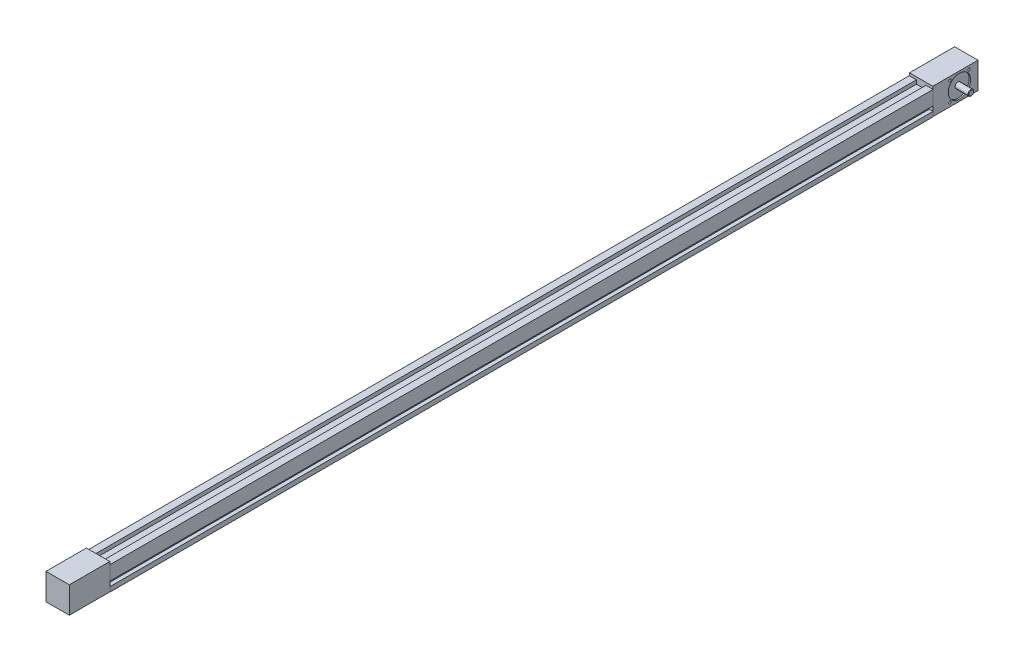
SolidWorks part; units mm, degrees
ref_plane "前视" through (0, 0, 0) normal (0, 0, 1) x (1, 0, 0)
ref_plane "上视" through (0, 0, 0) normal (0, 1, 0) x (1, 0, 0)
ref_plane "右视" through (0, 0, 0) normal (1, 0, 0) x (0, 0, -1)
sketch "草图1" plane through (0, 0, 0) normal (0, 0, 1) x (1, 0, 0)
  line L0 (15, 50) -> (15, 42)
  line L1 (0, 0) -> (50, 0)
  line L2 (0, 0) -> (0, 10)
  line L3 (0, 50) -> (15, 50)
  line L4 (50, 0) -> (50, 10)
  line L5 (15, 42) -> (35, 42)
  line L6 (35, 42) -> (35, 50)
  line L7 (35, 50) -> (50, 50)
  line L8 (0, 20) -> (8, 20)
  line L10 (0, 10) -> (8, 10)
  line L11 (8, 20) -> (8, 10)
  line L12 (50, 20) -> (42, 20)
  line L13 (0, 20) -> (0, 50)
  line L14 (50, 10) -> (42, 10)
  line L15 (42, 20) -> (42, 10)
  line L16 (50, 20) -> (50, 50)
  dimension "D1" = 50
  dimension "D2" = 50
  dimension "D3" = 8
  dimension "D4" = 10
  dimension "D5" = 10
  dimension "D6" = 10
  dimension "D7" = 10
  dimension "D8" = 8
  dimension "D9" = 20
  dimension "D10" = 15
  dimension "D11" = 8
extrude "基体-拉伸" add sketch "草图1" along normal blind 1730
sketch "草图2" plane through (0, 0, 1730) normal (0, 0, 1) x (1, 0, 0)
  line L0 (0, 0) -> (50, 0) construction
  line L1 (0.5, 0) -> (49.5, 0)
  line L2 (0.5, 0) -> (0.5, 55.5)
  line L3 (0.5, 55.5) -> (49.5, 55.5)
  line L4 (49.5, 0) -> (49.5, 55.5)
  line L5 (0, 10) -> (0, 0) construction
  line L6 (50, 0) -> (50, 10) construction
  dimension "D1" = 55.5
  dimension "D2" = 0.5
  dimension "D3" = 0.5
extrude "凸台-拉伸1" add sketch "草图2" along normal blind 85
sketch "草图4" plane through (0, 0, 0) normal (0, 0, -1) x (-1, 0, 0)
  line L0 (-49.5, 50) -> (-49.5, 55.5) construction
  line L1 (-0.5, 0) -> (-49.5, 0)
  line L2 (-0.5, 0) -> (-0.5, 55.5)
  line L3 (-0.5, 55.5) -> (-49.5, 55.5)
  line L4 (-49.5, 0) -> (-49.5, 55.5)
  line L5 (-49.5, 55.5) -> (-0.5, 55.5) construction
extrude "凸台-拉伸3" add sketch "草图4" along normal blind 95
sketch "草图9" plane through (49.5, 0, 0) normal (1, 0, 0) x (0, 0, -1)
  line L0 (-1815, 0) -> (95, 0) construction
  line L3 (95, 55.5) -> (95, 0) construction
  circle A0 centre (56, 27.75) radius 23.5
  dimension "D3" = 47
  dimension "D1" = 39
  dimension "D2" = 27.75
extrude "切除-拉伸5" cut sketch "草图9" against normal blind 3
sketch "草图10" plane through (46.5, 0, 0) normal (1, 0, 0) x (0, 0, -1)
  circle A0 centre (56, 27.75) radius 6
  dimension "D1" = 12
extrude "凸台-拉伸4" add sketch "草图10" along normal blind 28
chamfer "倒角1" distance 1 angle 45 1 edges at (74.5, 27.75, -62)
sketch "草图11" plane through (50, 0, 0) normal (1, 0, 0) x (0, 0, -1)
  line L0 (76, 47.75) -> (56, 27.75) construction
  line L1 (56, 27.75) -> (54.0318, 27.75) construction
  circle A0 centre (56, 27.75) radius 23.5 construction
  point P0 (76, 47.75)
  dimension "D1" = 45
  dimension "D2" = 20
hole_wizard "M5 螺纹孔1" positions "3D草图1" profile "草图12" tap size "M5" standard "GB"
sketch3d "3D草图1"
  point P0 (50, 47.75, -76)
sketch "草图12" plane through (50, 47.75, -76) normal (0, 1, 0) x (0, 0, -1)
  line L0 (0, 0) -> (0, 15.2618)
  line L1 (0, 15.2618) -> (2.1, 14)
  line L2 (2.1, 14) -> (2.1, 10)
  line L3 (2.1, 10) -> (2.5, 10)
  line L4 (2.5, 10) -> (2.5, 0)
  line L5 (2.5, 0) -> (0, 0)
  line L10 (0, 15.2618) -> (-2.1, 14) construction
  line L11 (0, -6.35) -> (0, 107.95) construction
  dimension "螺纹孔钻头直径" = 4.2
  dimension "螺纹孔钻头深度" = 14
  dimension "螺纹主直径" = 5
  dimension "螺纹深度" = 10
  dimension "导头角度" = 118
pattern_circular "阵列(圆周)1" count 4 over 360 about axis through (0, 27.75, -56) along (1, 0, 0) of "M5 螺纹孔1"
